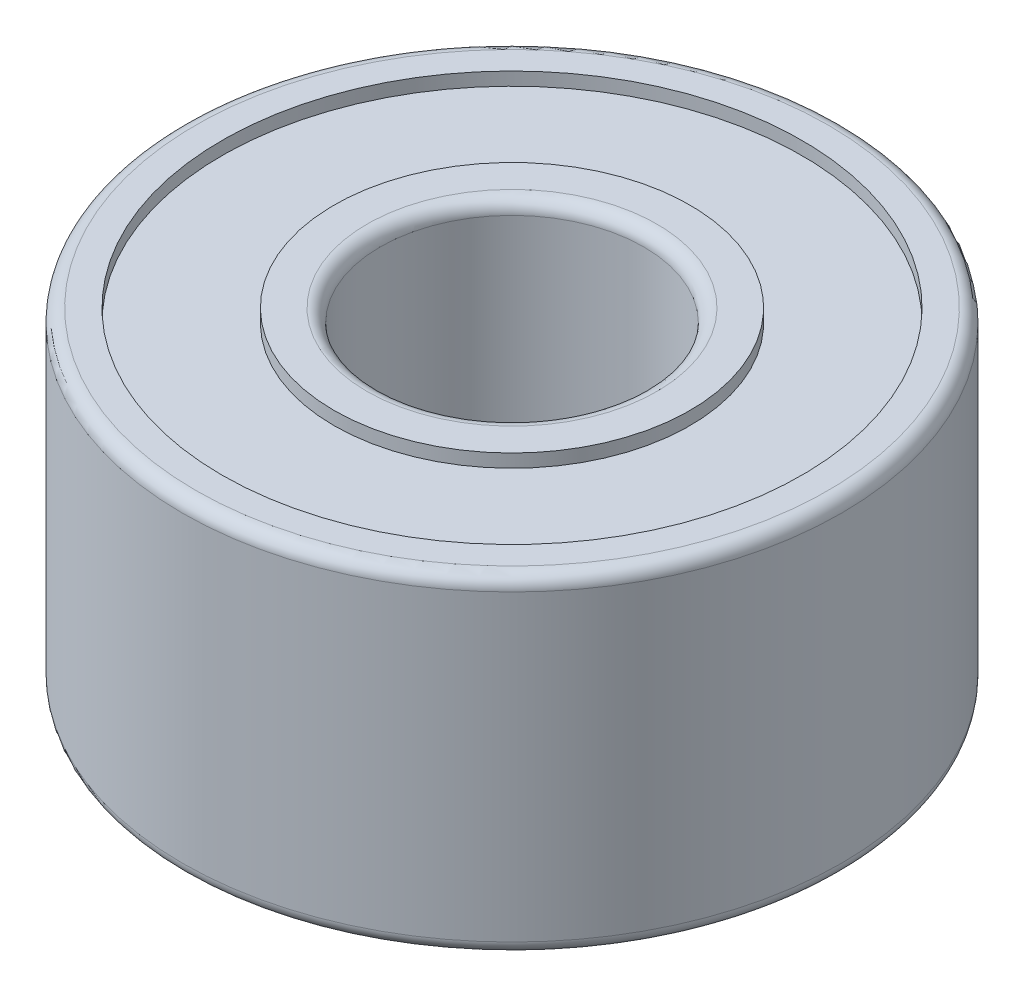
from build123d import *

# Parameters (mm, degrees)
SKETCH_1_R          = 2.5
SKETCH_1_R_2        = 1
EXTRUDE_1_DEPTH     = 2.5
SKETCH_2_R          = 2.2
SKETCH_2_R_2        = 1.35
CUT_EXTRUDE_1_DEPTH = 0.1
CUT_EXTRUDE_START   = -0.1
SKETCH_4_R          = 2.2
SKETCH_4_R_2        = 1.35
CUT_EXTRUDE_2_DEPTH = 0.1
FILLET_R0_1_1_R     = 0.1


with BuildPart() as part:
    # 草图1 → 凸台-拉伸1 (new body)
    with BuildSketch(Plane(origin=(0, 0, 0), x_dir=(1, 0, 0), z_dir=(0, 1, 0))):
        with Locations(Location((0, 0, 0), (0, 0, 270))):
            Circle(SKETCH_1_R)
        with Locations(Location((0, 0, 0), (0, 0, 270))):
            Circle(SKETCH_1_R_2, mode=Mode.SUBTRACT)
    extrude(amount=EXTRUDE_1_DEPTH)

    # 草图2 → 切除-拉伸1 (cut)
    with BuildSketch(Plane(origin=(0, 2.5, 0), x_dir=(1, 0, 0), z_dir=(0, 1, 0))):
        with Locations(Location((0, 0, 0), (0, 0, 270))):
            Circle(SKETCH_2_R)
        with Locations(Location((0, 0, 0), (0, 0, 270))):
            Circle(SKETCH_2_R_2, mode=Mode.SUBTRACT)
    extrude(amount=-CUT_EXTRUDE_1_DEPTH, mode=Mode.SUBTRACT)

    # 草图4 → 切除-拉伸2 (cut)
    with BuildSketch(Plane.XZ.offset(CUT_EXTRUDE_START)):
        with Locations(Location((0, 0, 0), (0, 0, 90))):
            Circle(SKETCH_4_R)
        with Locations(Location((0, 0, 0), (0, 0, 90))):
            Circle(SKETCH_4_R_2, mode=Mode.SUBTRACT)
    extrude(amount=CUT_EXTRUDE_2_DEPTH, mode=Mode.SUBTRACT)

    # R0.1 圆角1
    fillet_r0_1_1_edges = [part.edges().sort_by_distance(p)[0] for p in [
        (0, 0, -2.5),
        (0, 2.5, -2.5),
        (0, 0, -1),
        (0, 2.5, -1),
    ]]
    fillet(fillet_r0_1_1_edges, radius=FILLET_R0_1_1_R)


solid = part.part
